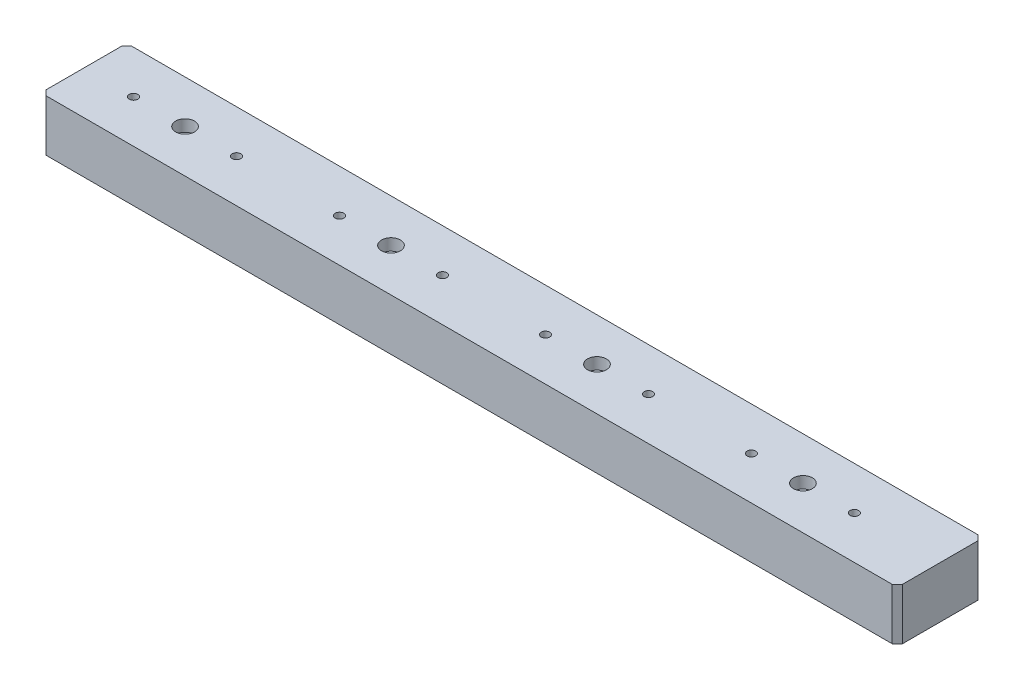
from build123d import *

# Parameters (mm, degrees)
SKETCH_1_W                = 499
SKETCH_1_H                = 50
EXTRUDE_1_DEPTH           = 30
CHAMFER_1_SIZE            = 3
HOLE_WIZARD_M6_1_D        = 5
HOLE_WIZARD_M6_1_DEPTH    = 15
HOLE_WIZARD_M6_1_TIP      = 1.502151548
HOLE_WIZARD_1_D           = 6.6
HOLE_WIZARD_1_DEPTH       = 30
HOLE_WIZARD_1_CBORE_D     = 11
HOLE_WIZARD_1_CBORE_DEPTH = 6.8
HOLE_WIZARD_1_TIP         = 1.982840043


with BuildPart() as part:
    # 草图1 → 凸台-拉伸1 (new body)
    with BuildSketch(Plane(origin=(0, 0, 0), x_dir=(1, 0, 0), z_dir=(0, 1, 0))):
        Rectangle(SKETCH_1_W, SKETCH_1_H)
    extrude(amount=EXTRUDE_1_DEPTH)

    # 倒角1
    chamfer_1_edges = [part.edges().sort_by_distance(p)[0] for p in [
        (249.5, 15, 25),
        (-249.5, 15, 25),
        (-249.5, 15, -25),
        (249.5, 15, -25),
    ]]
    chamfer(chamfer_1_edges, length=CHAMFER_1_SIZE)

    # M6 螺纹孔1
    with Locations(Plane(origin=(0, 30, 0), x_dir=(1, 0, 0), z_dir=(0, 1, 0))):
        with Locations((199.5, 0), (139.5, 0), (79.5, 0), (19.5, 0), (-40.5, 0), (-100.5, 0), (-160.5, 0), (-220.5, 0)):
            Hole(HOLE_WIZARD_M6_1_D / 2, depth=HOLE_WIZARD_M6_1_DEPTH)
            with Locations((0, 0, -(HOLE_WIZARD_M6_1_DEPTH + HOLE_WIZARD_M6_1_TIP / 2))):  # 118° drill point
                Cone(0, HOLE_WIZARD_M6_1_D / 2, HOLE_WIZARD_M6_1_TIP, mode=Mode.SUBTRACT)

    # 打孔尺寸(%根据)内六角圆柱头螺钉的类型1
    with Locations(Plane(origin=(0, 30, 0), x_dir=(1, 0, 0), z_dir=(0, 1, 0))):
        with Locations((169.5, 0), (49.5, 0), (-70.5, 0), (-190.5, 0)):
            CounterBoreHole(HOLE_WIZARD_1_D / 2, HOLE_WIZARD_1_CBORE_D / 2, HOLE_WIZARD_1_CBORE_DEPTH, depth=HOLE_WIZARD_1_DEPTH)
            with Locations((0, 0, -(HOLE_WIZARD_1_DEPTH + HOLE_WIZARD_1_TIP / 2))):  # 118° drill point
                Cone(0, HOLE_WIZARD_1_D / 2, HOLE_WIZARD_1_TIP, mode=Mode.SUBTRACT)


solid = part.part
